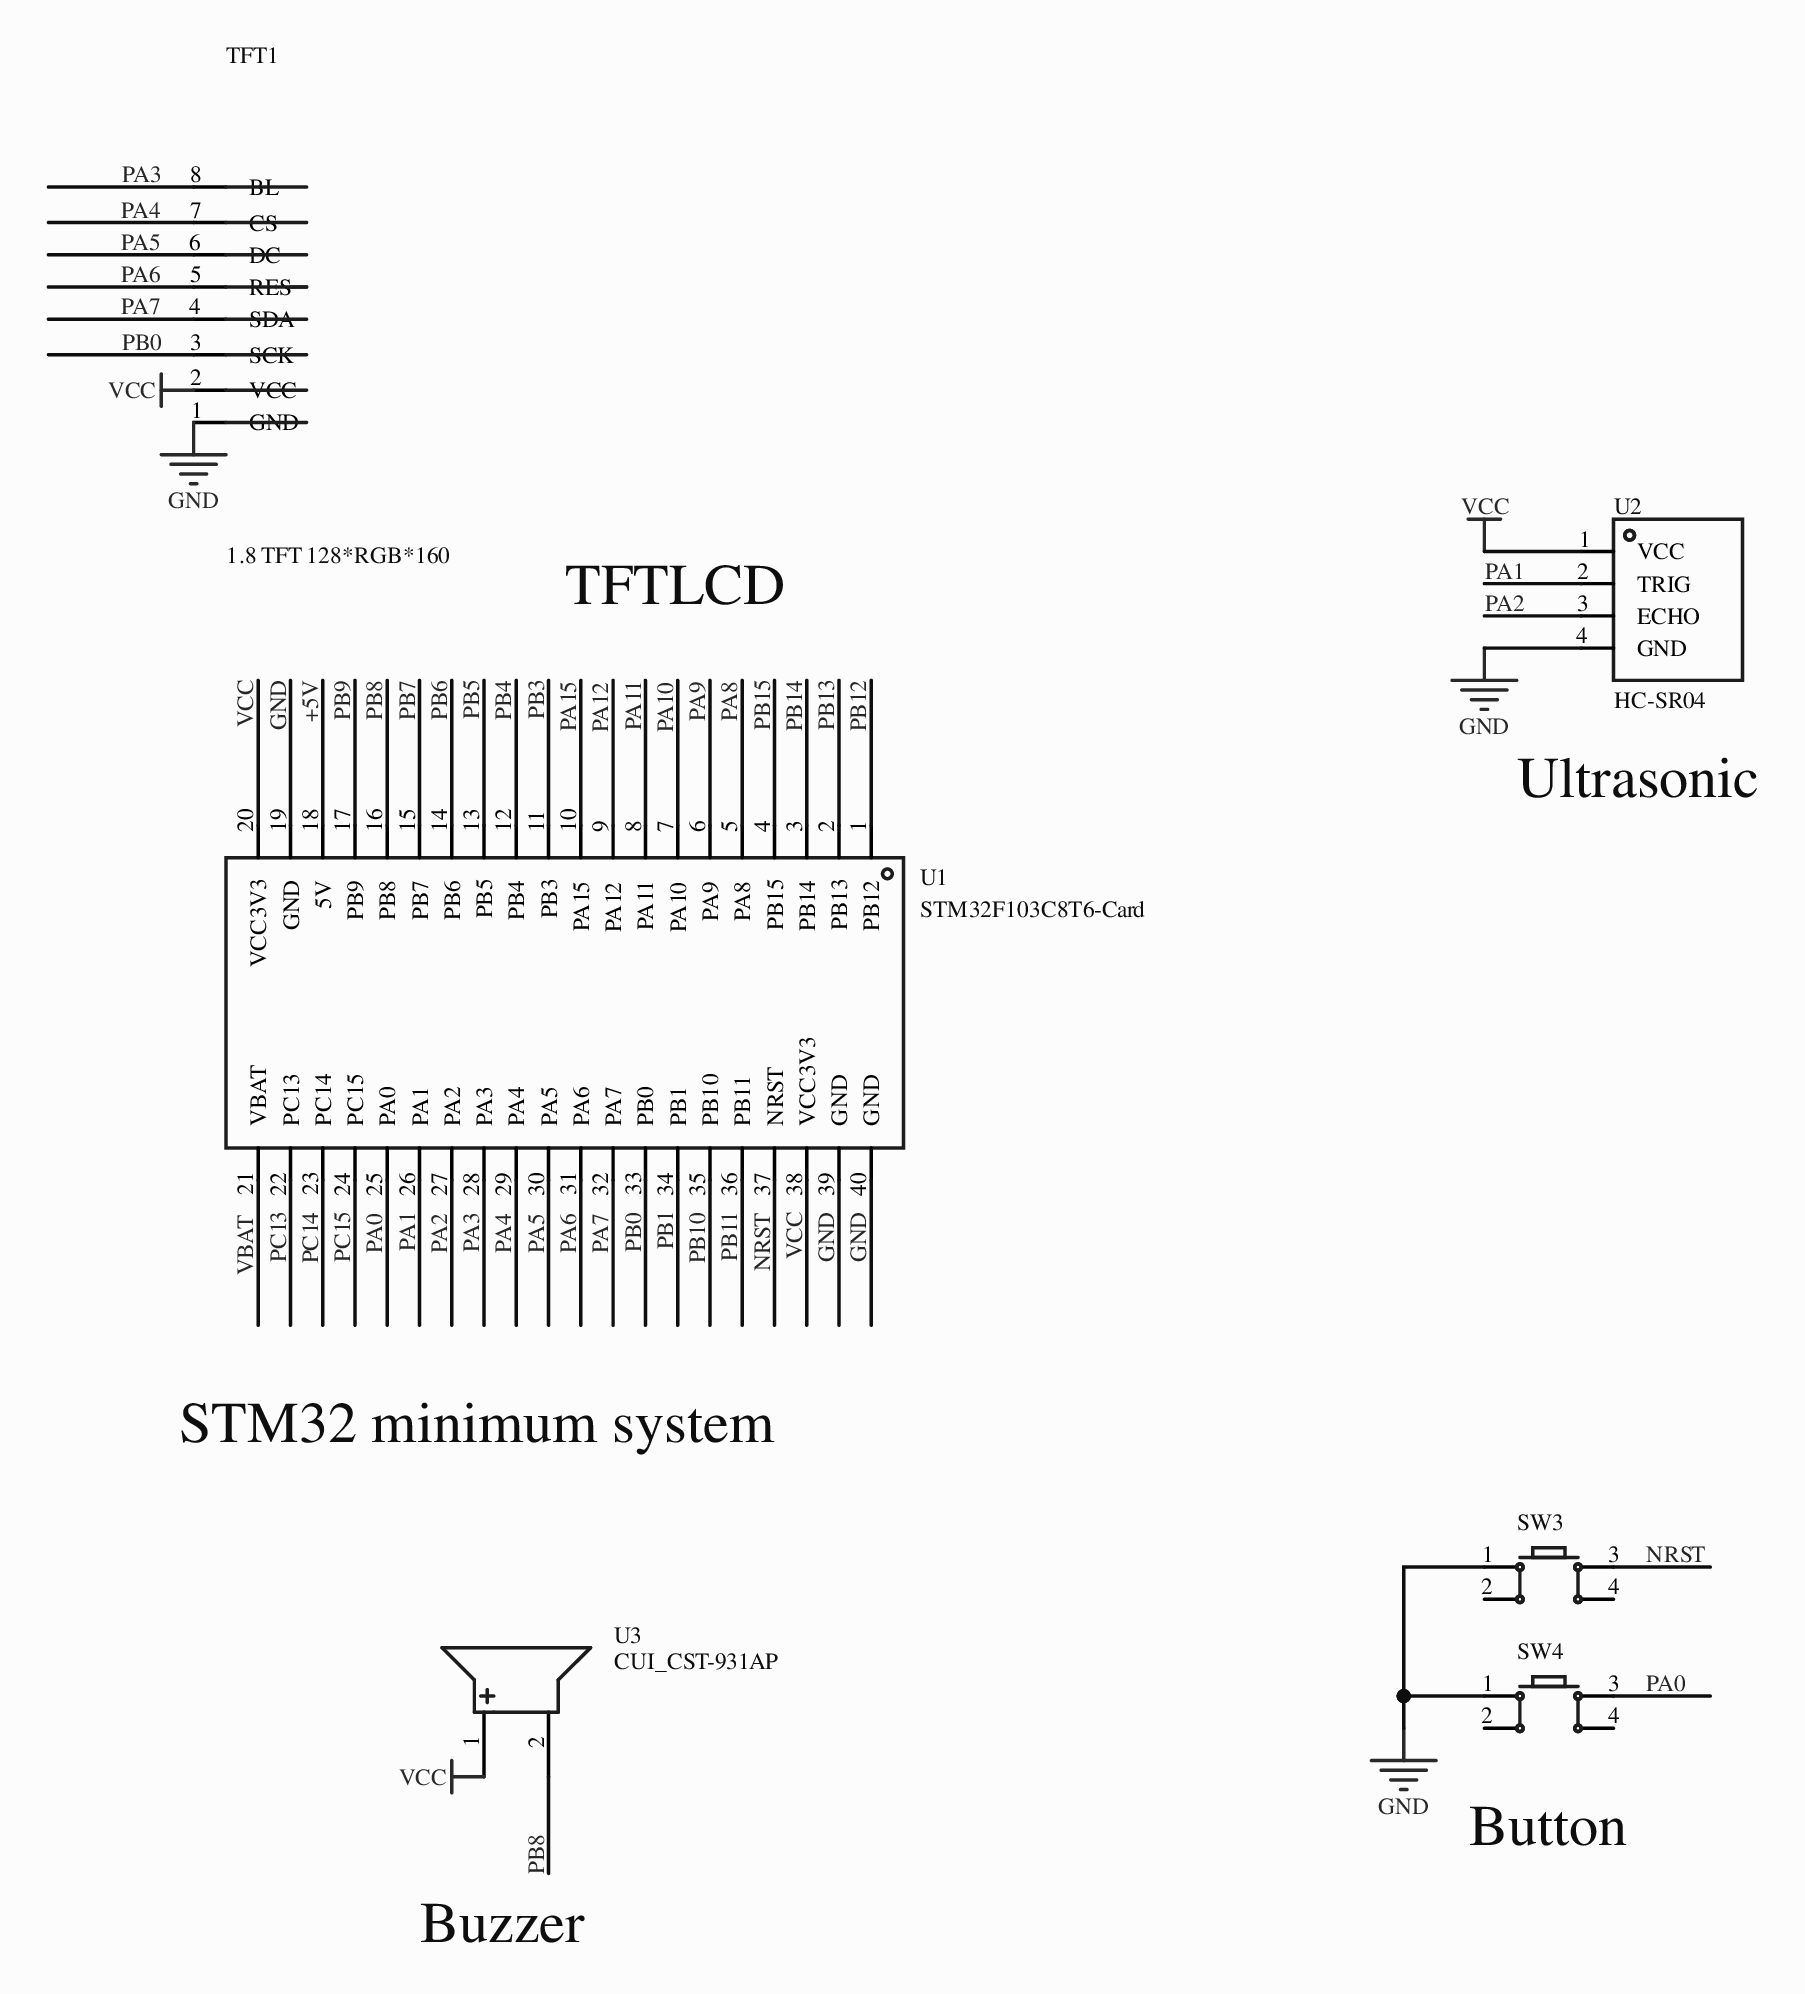
[diagram p0: MISC49920-3.schdoc]
# Altium project MISC49920-2.PrjPcb
1 sheet, 6 parts. Net scope: global (net labels, ports and power ports of the same name join across sheets).
Board file: MISC49920.pcbdoc

## Sheet MISC49920-3.schdoc
size 297 x 209 mm; Version: V1.0; @Project Name: MISC49920; @Page Count: 1; @Update Date: 2026-04-19; @Create Date: 2026-04-19; @Schematic Name: MISC49920; @Page No: 1; @Create Time: 23:22:16; @Update Time: 17:32:40; @Board Name: MISC49920

### Parts
SW3  (no value)  [SW-TH_4P-L6.0-W6.0-P4.50-LS6.5]
SW4  (no value)  [SW-TH_4P-L6.0-W6.0-P4.50-LS6.5]
TFT1  1.8 TFT 128*RGB*160  [LCD-TH_8P-P2.54-L56.0-W34.0_1.8-TFT]
U1  STM32F103C8T6-Card  [CONN-TH_L53.3-W22.9_STM32F103C8T6-CARD]
U2  HC-SR04  [TH_HC-SR04V]
U3  CUI_CST-931AP  [BUZ-TH_BD9.0-P4.00-D0.6-L-FD]

### Nets
GND: SW3.1 SW4.1 TFT1.1(GND) U1.19(GND) U1.39(GND) U1.40(GND) U2.4(GND)
VCC: TFT1.2(VCC) U1.20(VCC3V3) U1.38(VCC3V3) U2.1(VCC) U3.1
+5V: U1.18(5V)
NRST: SW3.3 U1.37(NRST)
PA0: SW4.3 U1.25(PA0)
PA1: U1.26(PA1) U2.2(TRIG)
PA2: U1.27(PA2) U2.3(ECHO)
PA3: TFT1.8(BL) U1.28(PA3)
PA4: TFT1.7(CS) U1.29(PA4)
PA5: TFT1.6(DC) U1.30(PA5)
PA6: TFT1.5(RES) U1.31(PA6)
PA7: TFT1.4(SDA) U1.32(PA7)
PA8: U1.5(PA8)
PA9: U1.6(PA9)
PA10: U1.7(PA10)
PA11: U1.8(PA11)
PA12: U1.9(PA12)
PA15: U1.10(PA15)
PB0: TFT1.3(SCK) U1.33(PB0)
PB1: U1.34(PB1)
PB3: U1.11(PB3)
PB4: U1.12(PB4)
PB5: U1.13(PB5)
PB6: U1.14(PB6)
PB7: U1.15(PB7)
PB8: U1.16(PB8) U3.2
PB9: U1.17(PB9)
PB10: U1.35(PB10)
PB11: U1.36(PB11)
PB12: U1.1(PB12)
PB13: U1.2(PB13)
PB14: U1.3(PB14)
PB15: U1.4(PB15)
PC13: U1.22(PC13)
PC14: U1.23(PC14)
PC15: U1.24(PC15)
VBAT: U1.21(VBAT)

Not connected (* = marked no-connect by the designer): SW3 2 4; SW4 2 4

### Notes on the sheet
- TFTLCD
- (near U2) Ultrasonic
- STM32 minimum system
- (near SW4) Button
- Buzzer

### Library data of the parts
SW3 SW4 = Key_TH_6x6x6: Contact current:50mA;Rated voltage(DC):12V;Insulation resistance:100MΩ;Circuit structure:SPST;Mounting:through-hole;Button shape:round button;Button/cap colour:black;Actuation force:260gf@±30gf;Operating temperature:-25℃~+70℃;Pin style:PC pin;Switch length:6mm;Switch width:6mm;Switch height:6mm;With bracket:no;; Symbol: Tactile button; AddInBom: yes; ModelId: 20eee248bc684ccd8cbdbb1d0d91ec6f0819f05c4eef4c71ace90d822a990e87; ModelName: SW-TH_4P-L6.0-W6.0-H5.0-LS6.5-P4.50; ModelTransform: 236.22,323.03,0,90,0,0,0,0,-137.795; Device: Key_TH_6x6x6; FootprintName: SW-TH_4P-L6.0-W6.0-P4.50-LS6.5; ConvertToPcb: yes; Supplier Footprint: 插件
TFT1 = 1.8 TFT 128*RGB*160: AddInBom: yes; Symbol: 1.8 TFT 128*RGB*160; Device: 1.8 TFT 128*RGB*160; LCSC Part Name: 1.8 TFT 128*RGB*160; SupplierPart: C9900080251; ManufacturerPart: 1.8 TFT 128*RGB*160; Supplier Footprint: 插件; Supplier: LCSC; ConvertToPcb: yes; FootprintName: LCD-TH_8P-P2.54-L56.0-W34.0_1.8-TFT
U1 = STM32F103C8T6-Card: AddInBom: yes; Device: STM32F103C8T6-Card; Symbol: STM32F103C8T6-CARD; FootprintName: CONN-TH_L53.3-W22.9_STM32F103C8T6-CARD; LCSC Part Name: STM32F103C8T6-Card; SupplierPart: C9900077949; ManufacturerPart: STM32F103C8T6-Card; Supplier Footprint: 插件; Supplier: LCSC; ConvertToPcb: yes
U2 = HC-SR04: Manufacturer: Universal Microelectronics; AddInBom: yes; Symbol: HC-SR04; Device: HC-SR04; LCSC Part Name: HC-SR04; SupplierPart: C19857336; ManufacturerPart: HC-SR04; Supplier Footprint: -; JLCPCB Part Class: Extended library; Datasheet: https://example.com/upload/public/pdf/source/20240122/47B8E374E428935B7962A2189EF91AAC.pdf; Supplier: LCSC; ConvertToPcb: yes; FootprintName: TH_HC-SR04V
U3 = CUI_CST-931AP: AddInBom: yes; ModelId: 4783197d75f9410a8852901e7a7769db0819f05c4eef4c71ace90d822a990e87; ModelTransform: 354.33,354.33,0,270,0,0,0,0,-196.85; Symbol: CUI_CST-931AP; Device: CUI_CST-931AP; LCSC Part Name: CUI_CST-931AP; SupplierPart: C9900006511; ManufacturerPart: CUI_CST-931AP; Supplier Footprint: BUZZERPIEZO3V30MMTH; JLCPCB Part Class: Extended Part; Supplier: LCSC; ConvertToPcb: yes; FootprintName: BUZ-TH_BD9.0-P4.00-D0.6-L-FD; ModelName: BUZ-TH_BD9.0-P4.00-D0.6-L-FD